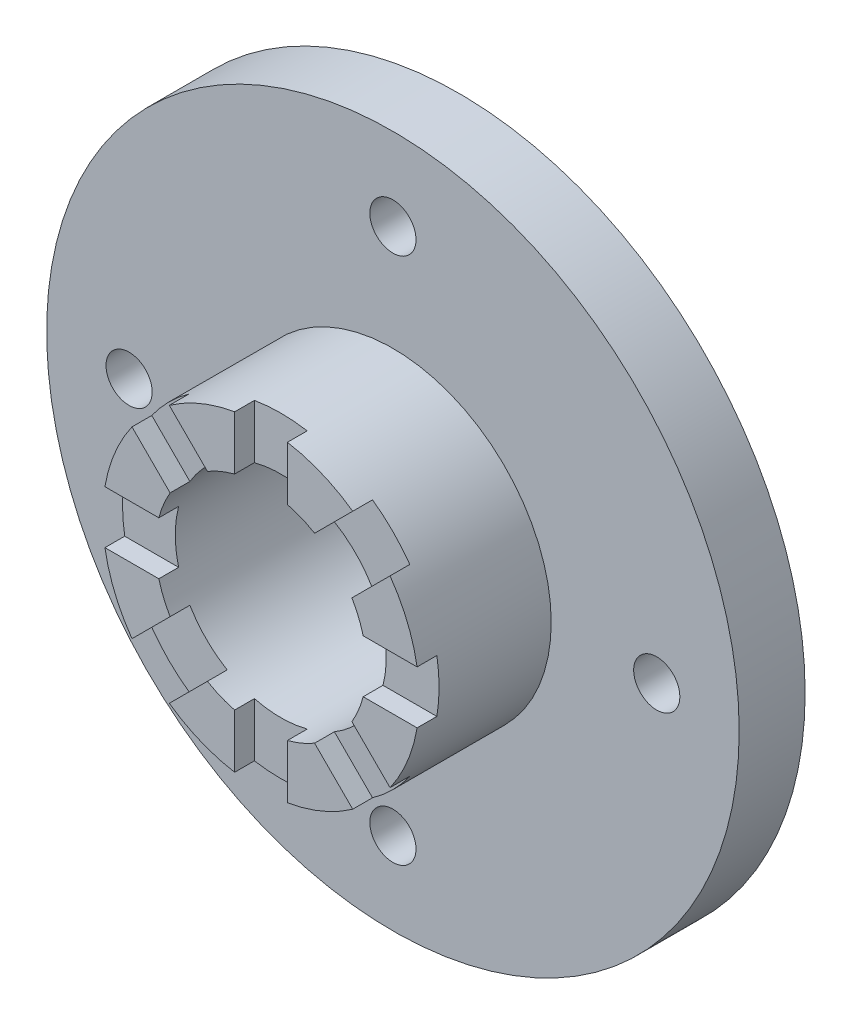
from build123d import *

# Parameters (mm, degrees)
SKETCH_1_R          = 52.5
SKETCH_1_R_2        = 16
SKETCH_1_R_3        = 3.5
EXTRUDE_1_DEPTH     = 10
SKETCH_2_R          = 24
SKETCH_2_R_2        = 16
EXTRUDE_2_DEPTH     = 20
CUT_EXTRUDE_START   = -3
CUT_EXTRUDE_2_DEPTH = 3


with BuildPart() as part:
    # 草图1 → 凸台-拉伸1 (new body)
    with BuildSketch(Plane.XY):
        Circle(SKETCH_1_R)
        Circle(SKETCH_1_R_2, mode=Mode.SUBTRACT)
        with Locations((0, 40)):
            Circle(SKETCH_1_R_3, mode=Mode.SUBTRACT)
        with Locations((40, 0)):
            Circle(SKETCH_1_R_3, mode=Mode.SUBTRACT)
        with Locations((0, -40)):
            Circle(SKETCH_1_R_3, mode=Mode.SUBTRACT)
        with Locations((-40, 0)):
            Circle(SKETCH_1_R_3, mode=Mode.SUBTRACT)
    extrude(amount=EXTRUDE_1_DEPTH)

    # 草图2 → 凸台-拉伸2 (add)
    with BuildSketch(Plane.XY.offset(10)):
        Circle(SKETCH_2_R)
        Circle(SKETCH_2_R_2, mode=Mode.SUBTRACT)
    extrude(amount=EXTRUDE_2_DEPTH)

    # 草图3 → 切除-拉伸2 (cut)
    with BuildSketch(Plane.XY.offset(30).offset(CUT_EXTRUDE_START)):
        with BuildLine():
            Line((-4, 23.664319132), (-4, 15.491933385))
            ThreePointArc((-4, 15.491933385), (0, 16), (4, 15.491933385))
            Line((4, 15.491933385), (4, 23.664319132))
            ThreePointArc((4, 23.664319132), (0, 24), (-4, 23.664319132))
        make_face()
        with BuildLine():
            Line((13.904773406, 19.561627655), (8.126024025, 13.782878275))
            ThreePointArc((8.126024025, 13.782878275), (11.313708499, 11.313708499), (13.782878275, 8.126024025))
            Line((13.782878275, 8.126024025), (19.561627655, 13.904773406))
            ThreePointArc((19.561627655, 13.904773406), (16.970562748, 16.970562748), (13.904773406, 19.561627655))
        make_face()
        with BuildLine():
            Line((23.664319132, 4), (15.491933385, 4))
            ThreePointArc((15.491933385, 4), (16, 0), (15.491933385, -4))
            Line((15.491933385, -4), (23.664319132, -4))
            ThreePointArc((23.664319132, -4), (24, 0), (23.664319132, 4))
        make_face()
        with BuildLine():
            Line((19.561627655, -13.904773406), (13.782878275, -8.126024025))
            ThreePointArc((13.782878275, -8.126024025), (11.313708499, -11.313708499), (8.126024025, -13.782878275))
            Line((8.126024025, -13.782878275), (13.904773406, -19.561627655))
            ThreePointArc((13.904773406, -19.561627655), (16.970562748, -16.970562748), (19.561627655, -13.904773406))
        make_face()
        with BuildLine():
            Line((4, -23.664319132), (4, -15.491933385))
            ThreePointArc((4, -15.491933385), (0, -16), (-4, -15.491933385))
            Line((-4, -15.491933385), (-4, -23.664319132))
            ThreePointArc((-4, -23.664319132), (0, -24), (4, -23.664319132))
        make_face()
        with BuildLine():
            Line((-13.904773406, -19.561627655), (-8.126024025, -13.782878275))
            ThreePointArc((-8.126024025, -13.782878275), (-11.313708499, -11.313708499), (-13.782878275, -8.126024025))
            Line((-13.782878275, -8.126024025), (-19.561627655, -13.904773406))
            ThreePointArc((-19.561627655, -13.904773406), (-16.970562748, -16.970562748), (-13.904773406, -19.561627655))
        make_face()
        with BuildLine():
            Line((-23.664319132, -4), (-15.491933385, -4))
            ThreePointArc((-15.491933385, -4), (-16, 0), (-15.491933385, 4))
            Line((-15.491933385, 4), (-23.664319132, 4))
            ThreePointArc((-23.664319132, 4), (-24, 0), (-23.664319132, -4))
        make_face()
        with BuildLine():
            Line((-19.561627655, 13.904773406), (-13.782878275, 8.126024025))
            ThreePointArc((-13.782878275, 8.126024025), (-11.313708499, 11.313708499), (-8.126024025, 13.782878275))
            Line((-8.126024025, 13.782878275), (-13.904773406, 19.561627655))
            ThreePointArc((-13.904773406, 19.561627655), (-16.970562748, 16.970562748), (-19.561627655, 13.904773406))
        make_face()
    extrude(amount=CUT_EXTRUDE_2_DEPTH, mode=Mode.SUBTRACT)


solid = part.part
